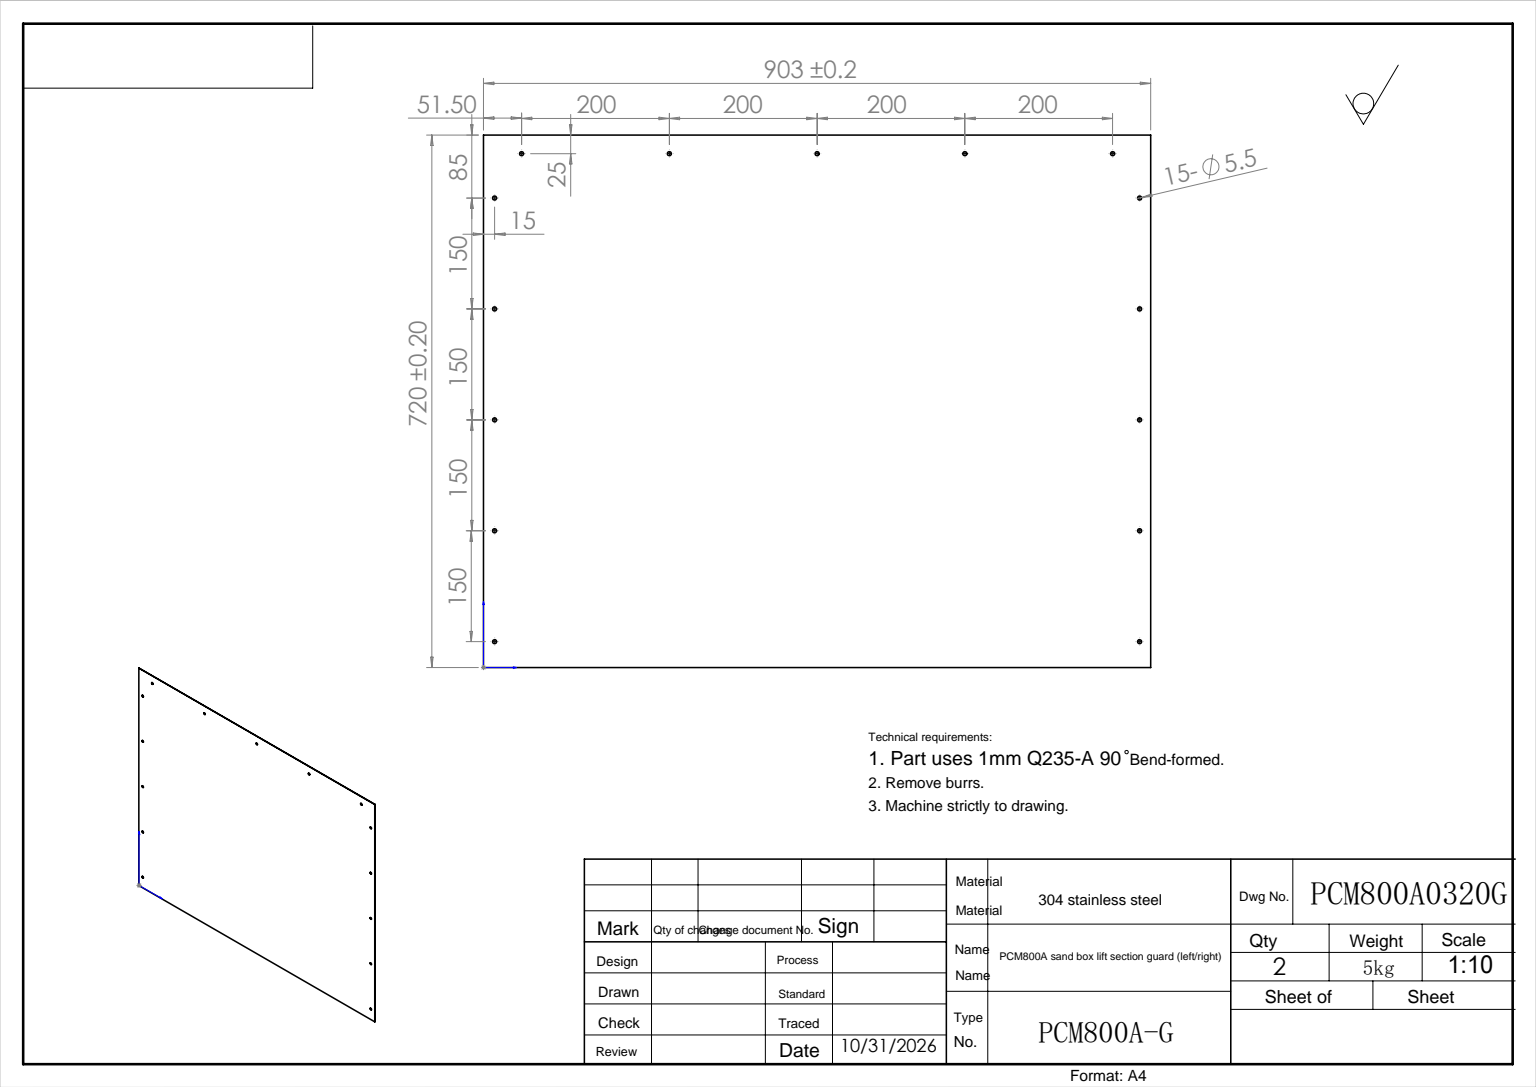
SolidWorks part; units mm, degrees
ref_plane "前视基准面" through (0, 0, 0) normal (0, 0, 1) x (1, 0, 0)
ref_plane "上视基准面" through (0, 0, 0) normal (0, 1, 0) x (1, 0, 0)
ref_plane "右视基准面" through (0, 0, 0) normal (1, 0, 0) x (0, 0, -1)
sketch "草图1" plane through (0, 0, 0) normal (0, 0, 1) x (1, 0, 0)
  line L1 (0, 0) -> (903, 0)
  line L2 (0, 0) -> (0, 720)
  line L3 (0, 720) -> (903, 720)
  line L4 (903, 0) -> (903, 720)
  dimension "D1" = 720
  dimension "D2" = 903
extrude "凸台-拉伸1" add sketch "草图1" along normal blind 1
sketch "草图2" plane through (0, 0, 1) normal (0, 0, 1) x (1, 0, 0)
  line L0 (0, 720) -> (0, 0) construction
  line L1 (903, 720) -> (0, 720) construction
  line L4 (0, 0) -> (903, 0) construction
  line L5 (451.5, 0) -> (451.5, 836.3556) construction
  circle A0 centre (51.5, 695) radius 2.75
  circle A1 centre (15, 635) radius 2.75
  circle A2 centre (251.5, 695) radius 2.75
  circle A3 centre (451.5, 695) radius 2.75
  circle A4 centre (651.5, 695) radius 2.75
  circle A5 centre (851.5, 695) radius 2.75
  circle A6 centre (15, 485) radius 2.75
  circle A7 centre (15, 335) radius 2.75
  circle A8 centre (15, 185) radius 2.75
  circle A9 centre (15, 35) radius 2.75
  circle A10 centre (888, 35) radius 2.75
  circle A11 centre (888, 185) radius 2.75
  circle A12 centre (888, 335) radius 2.75
  circle A13 centre (888, 485) radius 2.75
  circle A14 centre (888, 635) radius 2.75
  dimension "D3" = 5.5
  dimension "D5" = 5.5
  dimension "D7" = 85
  dimension "D1" = 51.5
  dimension "D2" = 25
  dimension "D6" = 15
  dimension "D4" = 5
  dimension "D8" = 5
extrude "切除-拉伸1" cut sketch "草图2" against normal blind 1.5
